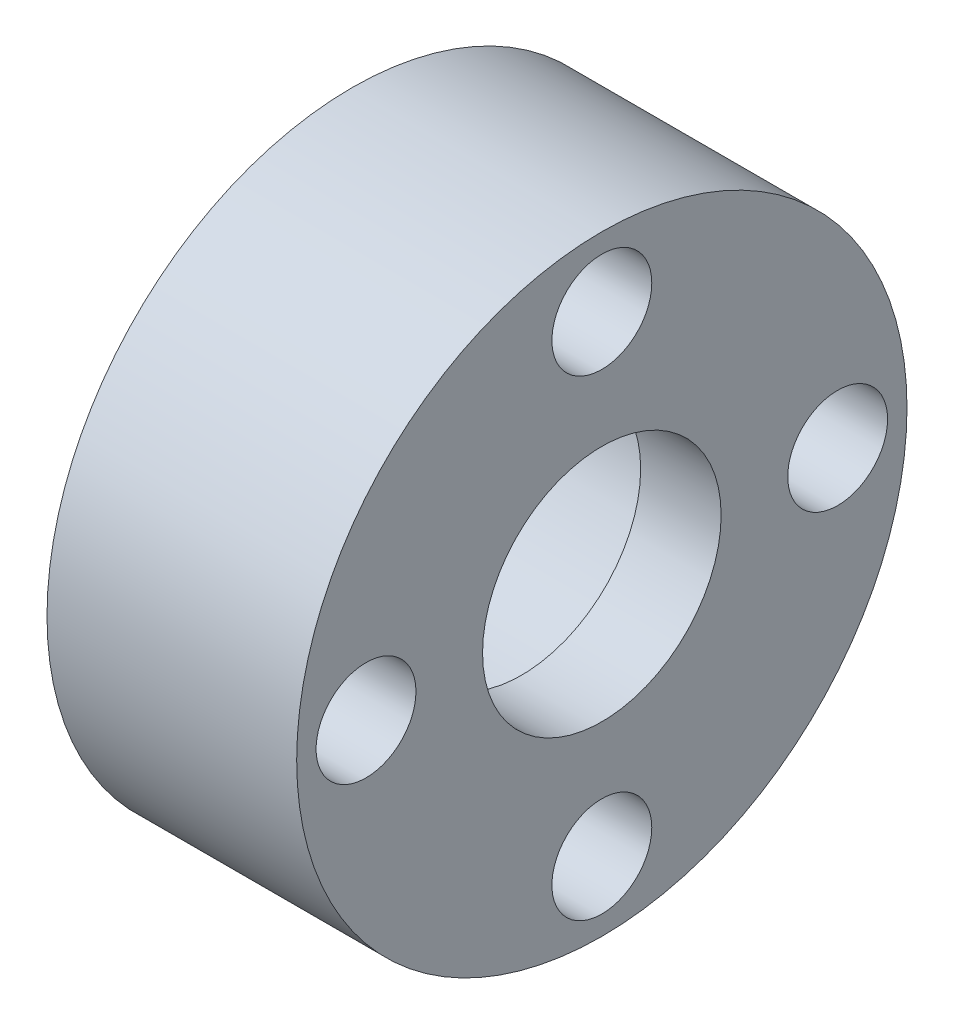
SolidWorks part; units mm, degrees
ref_plane "Front Plane" through (0, 0, 0) normal (0, 0, 1) x (1, 0, 0)
ref_plane "Top Plane" through (0, 0, 0) normal (0, 1, 0) x (1, 0, 0)
ref_plane "Right Plane" through (0, 0, 0) normal (1, 0, 0) x (0, 0, -1)
sketch "Sketch1" plane through (0, 0, 0) normal (0, 0, 1) x (1, 0, 0)
  line L0 (0, 0) -> (84.3025, 0) construction
  line L2 (48.9148, 21.5) -> (63.4148, 21.5)
  line L3 (18.4148, 30) -> (18.4148, 55)
  line L4 (18.4148, 55) -> (63.4148, 55)
  line L5 (63.4148, 21.5) -> (63.4148, 55)
  line L7 (48.9148, 21.5) -> (48.9148, 30)
  line L8 (48.9148, 30) -> (18.4148, 30)
  dimension "D1" = 43
  dimension "D2" = 60
  dimension "D3" = 110
  dimension "D4" = 45
  dimension "D5" = 30.5
  dimension "D6" = 18.4148
revolve "Revolve1" add sketch "Sketch1" angle 360 about L0
hole_wizard "Hole size per socket head cap screw type1" positions "Sketch3" profile "Sketch2" counterbore size "M10" standard "GB" end condition through all
sketch "Sketch3" plane through (63.4148, 0, 0) normal (1, 0, 0) x (0, 0, -1)
  circle A1 centre (0, 0) radius 42.5 construction
  point P0 (0, 42.5)
  point P1 (0, -42.5)
  point P3 (-42.5, 0)
  point P5 (42.5, 0)
  dimension "D1" = 85
sketch "Sketch2" plane through (63.4148, 42.5, 0) normal (0, 1, 0) x (0, 0, -1)
  line L0 (0, 0) -> (0, 45)
  line L1 (0, 45) -> (5.5, 45)
  line L3 (5.5, 45) -> (5.5, 20)
  line L4 (5.5, 20) -> (9, 20)
  line L5 (9, 20) -> (9, 0)
  line L7 (9, 0) -> (0, 0)
  line L11 (0, -6.35) -> (0, 107.95) construction
  dimension "通孔孔直径" = 11
  dimension "通孔孔深度" = 45
  dimension "柱形沉头孔直径" = 18
  dimension "柱形沉头孔深度" = 20
